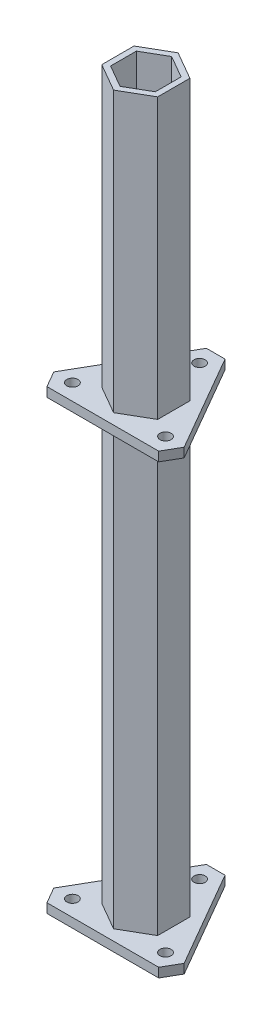
SolidWorks part; units mm, degrees
material "45"
ref_plane "Front Plane" through (0, 0, 0) normal (0, 0, 1) x (1, 0, 0)
ref_plane "Top Plane" through (0, 0, 0) normal (0, 1, 0) x (1, 0, 0)
ref_plane "Right Plane" through (0, 0, 0) normal (1, 0, 0) x (0, 0, -1)
sketch "Sketch1" plane through (0, 0, 0) normal (0, 1, 0) x (1, 0, 0)
  line L0 (-12, 6.9282) -> (-12, -6.9282)
  line L1 (0, 17.3205) -> (-15, 8.6603)
  line L2 (-15, 8.6603) -> (-15, -8.6603)
  line L3 (-15, -8.6603) -> (0, -17.3205)
  line L4 (0, -17.3205) -> (15, -8.6603)
  line L5 (15, -8.6603) -> (15, 8.6603)
  line L6 (15, 8.6603) -> (0, 17.3205)
  line L7 (-12, -6.9282) -> (0, -13.8564)
  line L8 (0, -13.8564) -> (12, -6.9282)
  line L9 (12, -6.9282) -> (12, 6.9282)
  line L10 (12, 6.9282) -> (0, 13.8564)
  line L11 (0, 13.8564) -> (-12, 6.9282)
  circle A0 centre (0, 0) radius 15 construction
  dimension "D1" = 30
  dimension "D2" = 3
extrude "Boss-Extrude1" add sketch "Sketch1" along normal mid plane 400
ref_plane "Plane1" through (0, 170, 0) normal (0, 1, 0) x (1, 0, 0)
sketch "Sketch2" plane through (0, 170, 0) normal (0, 1, 0) x (1, 0, 0)
  line L0 (15, 8.6603) -> (0, 17.3205) construction
  line L1 (15, -8.6603) -> (15, 8.6603) construction
  line L2 (0, -17.3205) -> (15, -8.6603) construction
  line L3 (-15, -8.6603) -> (0, -17.3205) construction
  line L4 (-15, 8.6603) -> (-15, -8.6603) construction
  line L5 (0, 17.3205) -> (-15, 8.6603) construction
  line L6 (15, 8.6603) -> (0, 17.3205)
  line L7 (15, -8.6603) -> (15, 8.6603)
  line L8 (0, -17.3205) -> (15, -8.6603)
  line L9 (-15, -8.6603) -> (0, -17.3205)
  line L10 (-15, 8.6603) -> (-15, -8.6603)
  line L11 (0, 17.3205) -> (-15, 8.6603)
  line L12 (0, 0) -> (0, 46.188) construction
  line L13 (0, 46.188) -> (-40, -23.094)
  line L14 (-40, -23.094) -> (40, -23.094)
  line L15 (40, -23.094) -> (0, 46.188)
  line L16 (-40, -23.094) -> (0, 0) construction
  line L17 (0, 0) -> (40, -23.094) construction
  dimension "D1" = 80
  dimension "D2" = 80
extrude "Boss-Extrude2" add sketch "Sketch2" against normal blind 5
sketch "Sketch3" plane through (0, 165, 0) normal (0, -1, 0) x (1, 0, 0)
  line L0 (0, 0) -> (0, 57.4818) construction
  line L1 (0, 0) -> (-40, 23.094) construction
  line L2 (0, 0) -> (40, 23.094) construction
  line L3 (0, -46.188) -> (40, 23.094)
  line L4 (40, 23.094) -> (-40, 23.094)
  line L5 (-40, 23.094) -> (0, -46.188)
  line L6 (0, -46.188) -> (5, -37.5278)
  line L7 (40, 23.094) -> (30, 23.094)
  line L8 (-40, 23.094) -> (-35, 14.4338)
  line L9 (-35, 14.4338) -> (-30, 23.094)
  line L10 (0, 0) -> (0, -46.188) construction
  line L11 (35, 14.4338) -> (30, 23.094)
  line L12 (-5, -37.5278) -> (5, -37.5278)
  line L13 (-5, -37.5278) -> (0, -46.188)
  line L14 (35, 14.4338) -> (40, 23.094)
  line L15 (-30, 23.094) -> (-40, 23.094)
  point P9 (-39.3478, 22.7175)
  point P14 (0, -41.7574)
  dimension "D2" = 10
  dimension "D1" = 0
extrude "Cut-Extrude1" cut sketch "Sketch3" against normal blind 5
pattern_linear "LPattern1" count 4 spacing 120 along (0, -1, 0) of "Boss-Extrude2", "Cut-Extrude1"
sketch "Sketch5" plane through (0, -195, 0) normal (0, -1, 0) x (1, 0, 0)
  line L3 (0, 0) -> (-40, 23.094) construction
  line L4 (0, 0) -> (40, 23.094) construction
  line L5 (0, 0) -> (0, -46.188) construction
  line L9 (-25, 14.4338) -> (0, 0) construction
  line L10 (0, 0) -> (0, -28.8675) construction
  line L11 (0, 0) -> (25, 14.4338) construction
  circle A0 centre (-25, 14.4338) radius 3
  circle A1 centre (25, 14.4338) radius 3
  circle A2 centre (0, -28.8675) radius 3
  circle A3 centre (0, 0) radius 28.8675 construction
  dimension "D1" = 6
  dimension "D2" = 120
  dimension "D3" = 50
extrude "Cut-Extrude2" cut sketch "Sketch5" against normal through all
sketch "Sketch7" plane through (0, 165, 0) normal (0, -1, 0) x (1, 0, 0)
  line L0 (-15, -8.6603) -> (-15, 8.6603) construction
  line L1 (-15, 8.6603) -> (0, 17.3205) construction
  line L2 (0, 17.3205) -> (15, 8.6603) construction
  line L3 (15, 8.6603) -> (15, -8.6603) construction
  line L4 (0, -17.3205) -> (-15, -8.6603) construction
  line L5 (15, -8.6603) -> (0, -17.3205) construction
  line L6 (30, 23.094) -> (-30, 23.094)
  line L7 (-30, 23.094) -> (-35, 14.4338)
  line L8 (-35, 14.4338) -> (-5, -37.5278)
  line L9 (-5, -37.5278) -> (5, -37.5278)
  line L10 (5, -37.5278) -> (35, 14.4338)
  line L11 (35, 14.4338) -> (30, 23.094)
  line L12 (30, 23.094) -> (-30, 23.094)
  line L13 (-30, 23.094) -> (-35, 14.4338)
  line L14 (-35, 14.4338) -> (-5, -37.5278)
  line L15 (-5, -37.5278) -> (5, -37.5278)
  line L16 (5, -37.5278) -> (35, 14.4338)
  line L17 (35, 14.4338) -> (30, 23.094)
  line L18 (-15, -8.6603) -> (-15, 8.6603)
  line L19 (-15, 8.6603) -> (0, 17.3205)
  line L20 (0, 17.3205) -> (15, 8.6603)
  line L21 (15, 8.6603) -> (15, -8.6603)
  line L22 (0, -17.3205) -> (-15, -8.6603)
  line L23 (15, -8.6603) -> (0, -17.3205)
  dimension "D1" = 0
extrude "Cut-Extrude4" cut sketch "Sketch7" against normal blind 10
sketch "Sketch8" plane through (0, -75, 0) normal (0, -1, 0) x (1, 0, 0)
  line L0 (0, 17.3205) -> (15, 8.6603) construction
  line L1 (15, 8.6603) -> (15, -8.6603) construction
  line L2 (15, -8.6603) -> (0, -17.3205) construction
  line L3 (0, -17.3205) -> (-15, -8.6603) construction
  line L4 (-15, -8.6603) -> (-15, 8.6603) construction
  line L5 (-15, 8.6603) -> (0, 17.3205) construction
  line L6 (-35, 14.4338) -> (-5, -37.5278)
  line L7 (-5, -37.5278) -> (5, -37.5278)
  line L8 (5, -37.5278) -> (35, 14.4338)
  line L9 (35, 14.4338) -> (30, 23.094)
  line L10 (30, 23.094) -> (-30, 23.094)
  line L11 (-30, 23.094) -> (-35, 14.4338)
  line L12 (-35, 14.4338) -> (-5, -37.5278)
  line L13 (-5, -37.5278) -> (5, -37.5278)
  line L14 (5, -37.5278) -> (35, 14.4338)
  line L15 (35, 14.4338) -> (30, 23.094)
  line L16 (30, 23.094) -> (-30, 23.094)
  line L17 (-30, 23.094) -> (-35, 14.4338)
  line L18 (0, 17.3205) -> (15, 8.6603)
  line L19 (15, 8.6603) -> (15, -8.6603)
  line L20 (15, -8.6603) -> (0, -17.3205)
  line L21 (0, -17.3205) -> (-15, -8.6603)
  line L22 (-15, -8.6603) -> (-15, 8.6603)
  line L23 (-15, 8.6603) -> (0, 17.3205)
  dimension "D1" = 0
extrude "Cut-Extrude5" cut sketch "Sketch8" against normal blind 10
